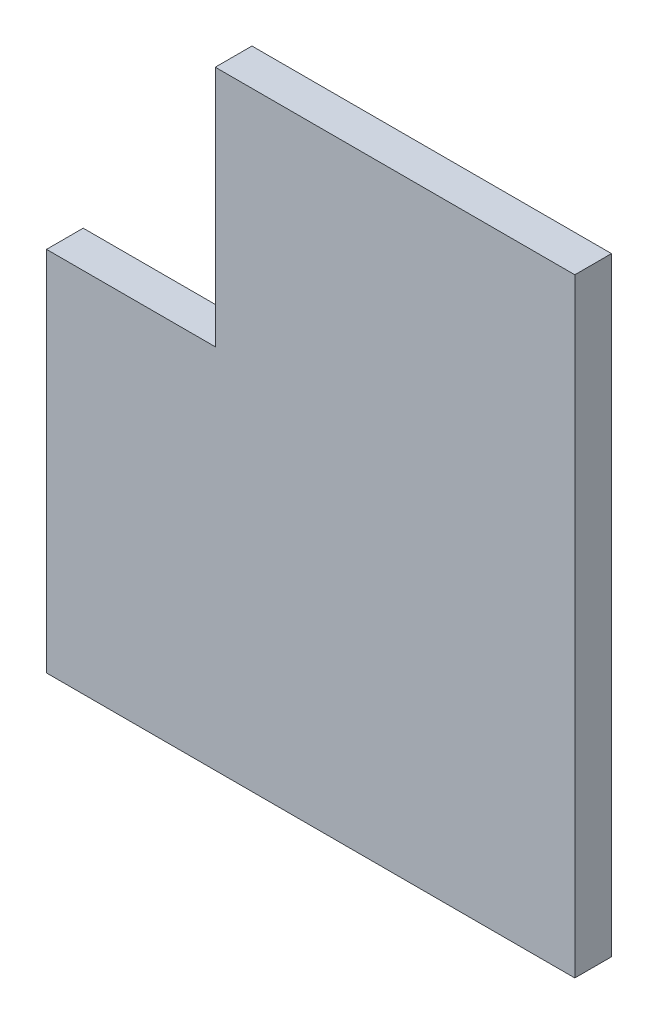
from build123d import *

# Parameters (mm, degrees)
BOSS_EXTRUDE1_DEPTH = 25


with BuildPart() as part:
    # Sketch1 → Boss-Extrude1 (new body)
    with BuildSketch(Plane.XY):
        Polygon((0, 0), (0, -415), (-360, -415), (-360, -165), (-245, -165), (-245, 0), align=None)
    extrude(amount=BOSS_EXTRUDE1_DEPTH)


solid = part.part
